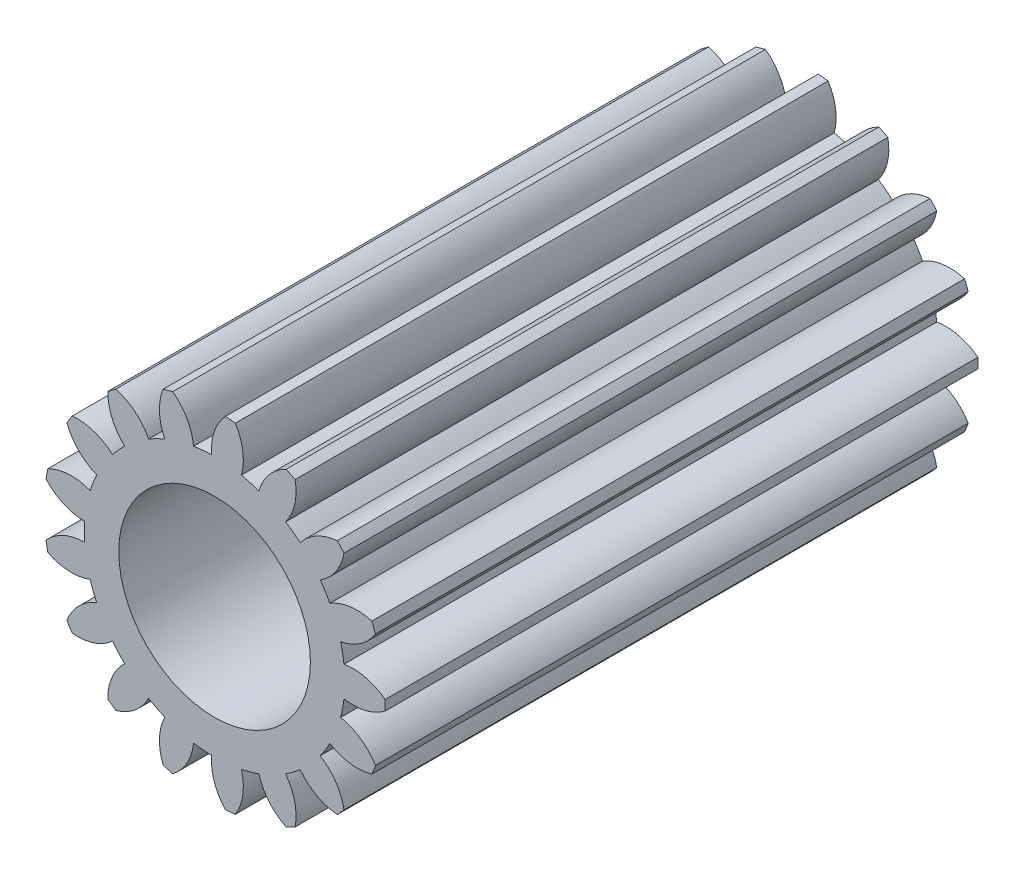
SolidWorks part; units mm, degrees
ref_plane "Front Plane" through (0, 0, 0) normal (0, 0, 1) x (1, 0, 0)
ref_plane "Top Plane" through (0, 0, 0) normal (0, 1, 0) x (1, 0, 0)
ref_plane "Right Plane" through (0, 0, 0) normal (1, 0, 0) x (0, 0, -1)
other "Configuration Table"
sketch "Sketch1" plane through (0, 0, 0) normal (0, 0, 1) x (1, 0, 0)
  circle A0 centre (0, 0) radius 10.875
  circle A1 centre (0, 0) radius 8
  dimension "D1" = 21.75
  dimension "D2" = 16
extrude "Boss-Extrude1" add sketch "Sketch1" along normal blind 49.5
sketch "Sketch2" plane through (0, 0, 49.5) normal (0, 0, 1) x (1, 0, 0)
  line L0 (0, 0) -> (0, 14.25) construction
  line L1 (0, 0) -> (4.8738, 13.3906) construction
  line L2 (0, 0) -> (1.3148, 14.1892) construction
  line L3 (0, 12.75) -> (4.0978, 11.2585) construction
  circle A0 centre (0, 0) radius 12.75 construction
  circle A1 centre (0, 0) radius 14.25
  circle A2 centre (0, 0) radius 10.875 construction
  circle A3 centre (0, 0) radius 10.875
  arc A4 (0.8984, 14.2217) -> (-0.2458, 10.8722) centre (4.0978, 11.2585) ccw
  arc A5 (1.7301, 14.1446) -> (2.2394, 10.6419) centre (-1.9592, 11.8198) cw
  dimension "D1" = 25.5
  dimension "D2" = 28.5
  dimension "D3" = 20
  dimension "D4" = 5.294
extrude "Boss-Extrude2" add sketch "Sketch2" against normal blind 49.5 contours A5 A1 A4 A3
pattern_circular "CirPattern1" count 17 over 360 about axis through (0, 0, 0) along (0, 0, 1) of "Boss-Extrude2"
